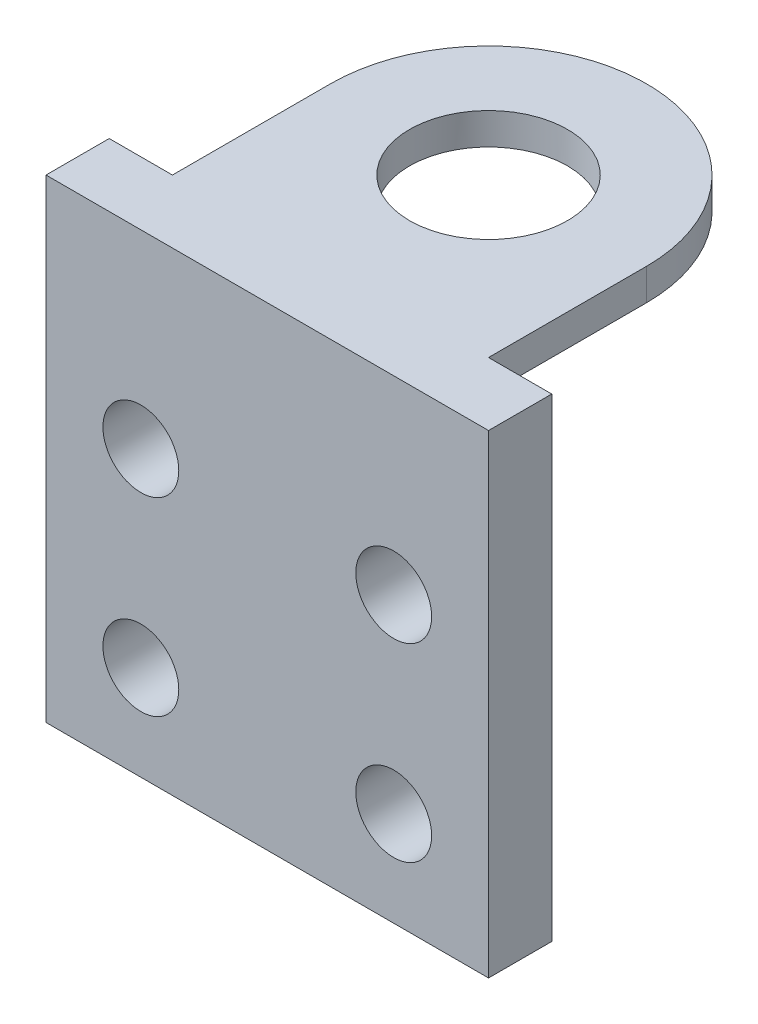
from build123d import *

# Parameters (mm, degrees)
SKETCH_1_W          = 70
SKETCH_1_H          = 70
SKETCH_1_R          = 6
EXTRUDE_1_DEPTH     = 10
SKETCH_2_W          = 70
SKETCH_2_H          = 5
EXTRUDE_2_DEPTH     = 60
SKETCH_4_R          = 12.5
CUT_EXTRUDE_1_DEPTH = 10


with BuildPart() as part:
    # 草图1 → 凸台-拉伸1 (new body)
    with BuildSketch(Plane.XY):
        with Locations((20, 20)):
            Rectangle(SKETCH_1_W, SKETCH_1_H)
        Circle(SKETCH_1_R, mode=Mode.SUBTRACT)
        with Locations((0, 30)):
            Circle(SKETCH_1_R, mode=Mode.SUBTRACT)
        with Locations((40, 30)):
            Circle(SKETCH_1_R, mode=Mode.SUBTRACT)
        with Locations((40, 0)):
            Circle(SKETCH_1_R, mode=Mode.SUBTRACT)
    extrude(amount=EXTRUDE_1_DEPTH)

    # 草图2 → 凸台-拉伸2 (add)
    with BuildSketch(Plane.XY.offset(10)):
        with Locations((20, 57.5)):
            Rectangle(SKETCH_2_W, SKETCH_2_H)
    extrude(amount=-EXTRUDE_2_DEPTH)

    # 草图4 → 切除-拉伸1 (cut)
    with BuildSketch(Plane(origin=(0, 60, 0), x_dir=(1, 0, 0), z_dir=(0, 1, 0))):
        with Locations(Location((20, 25, 0), (0, 0, 270))):
            Circle(SKETCH_4_R)
        with BuildLine():
            Line((-5, 25), (-5, 0))
            Line((-5, 0), (-23.267990544, 0))
            Line((-23.267990544, 0), (-23.267990544, 53.705684911))
            Line((-23.267990544, 53.705684911), (55, 53.705684911))
            Line((55, 53.705684911), (55, 0))
            Line((55, 0), (45, 0))
            Line((45, 0), (45, 25))
            ThreePointArc((45, 25), (20, 50), (-5, 25))
        make_face()
    extrude(amount=-CUT_EXTRUDE_1_DEPTH, mode=Mode.SUBTRACT)


solid = part.part
